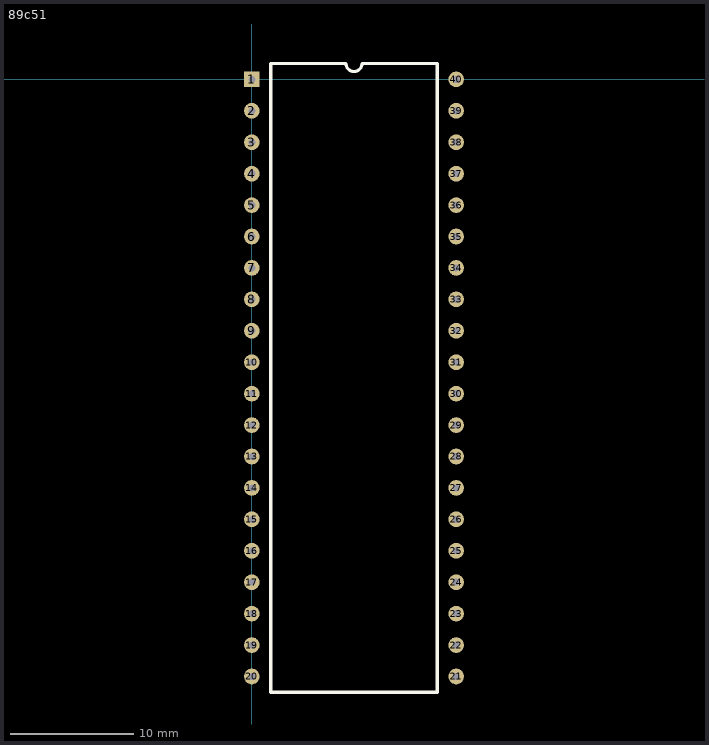
[diagram p0: the footprints below, top view; thin cyan lines are the x and y axes]
# Altium footprint library MISC89340-4.PcbLib: 4 footprints
Each footprint in its own frame and in the unit in brackets; x right, y up, seen from the top. Pads: shape width x height; smd on the part's side, far side on the other; paste and mask are expansions set on the pad; w line width, h text height; cw(c..) or ccw(c..) is an arc to the next point about the centre after c.

## 89c51 [mil]
pads (40):
  rect 50x50 hole 22: 1(0,0)
  round 50 hole 22: 2(0,-100) 3(0,-200) 4(0,-300) 5(0,-400) 6(0,-500) 7(0,-600) 8(0,-700) 9(0,-800) 10(0,-900) 11(0,-1000) 12(0,-1100) 13(0,-1200) 14(0,-1300) 15(0,-1400) 16(0,-1500) 17(0,-1600) 18(0,-1700) 19(0,-1800) 20(0,-1900) 21(650,-1900) 22(650,-1800) 23(650,-1700) 24(650,-1600) 25(650,-1500) 26(650,-1400) 27(650,-1300) 28(650,-1200) 29(650,-1100) 30(650,-1000) 31(650,-900) 32(650,-800) 33(650,-700) 34(650,-600) 35(650,-500) 36(650,-400) 37(650,-300) 38(650,-200) 39(650,-100) 40(650,0)
Top Overlay:
  lines w10: 60,-1950 60,50 300,50 ccw(c325,50) 350,50 590,50 590,-1950 60,-1950
3D body: height 190, standoff 35, extent 65,-1950 590,55

## PCBComponent_1 [mil]

## PCBComponent_1 - duplicate [mil]

## PCBComponent_1 - duplicate1 [mil]